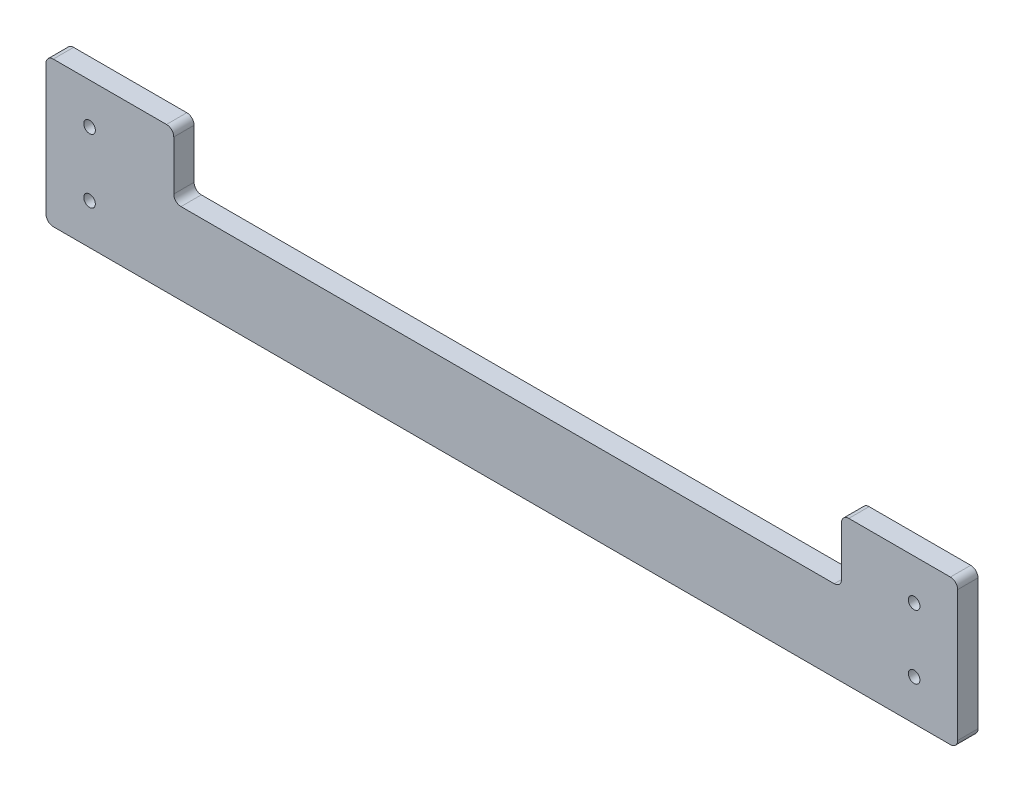
from build123d import *

# Parameters (mm, degrees)
SKETCH_1_W          = 1570
SKETCH_1_H          = 250
EXTRUDE_1_DEPTH     = 35
CUT_EXTRUDE_1_REACH = 797.66
SKETCH_2_W          = 1150
SKETCH_2_H          = 110
FILLET_1_R          = 12.5
CUT_EXTRUDE_2_REACH = 797.66
SKETCH_4_R          = 10


with BuildPart() as part:
    # 草图1 → 凸台-拉伸1 (new body)
    with BuildSketch(Plane.XY):
        Rectangle(SKETCH_1_W, SKETCH_1_H)
    extrude(amount=EXTRUDE_1_DEPTH)

    # 草图2 → 切除-拉伸1 (cut, up to next)
    with BuildSketch(Plane.XY.offset(35), mode=Mode.PRIVATE) as cut_extrude_1_sk1:
        with Locations((10, 70)):
            Rectangle(SKETCH_2_W, SKETCH_2_H)
    cut_extrude_1_tool1 = extrude(cut_extrude_1_sk1.sketch, amount=-CUT_EXTRUDE_1_REACH, mode=Mode.PRIVATE) & part.part
    add(cut_extrude_1_tool1.solids().sort_by_distance((10, 70, 35))[0], mode=Mode.SUBTRACT)

    # 圆角1
    fillet_1_edges = [part.edges().sort_by_distance(p)[0] for p in [
        (-565, 125, 17.5),
        (585, 125, 17.5),
        (585, 15, 17.5),
        (-565, 15, 17.5),
        (785, -125, 17.5),
        (-785, -125, 17.5),
        (-785, 125, 17.5),
        (785, 125, 17.5),
    ]]
    fillet(fillet_1_edges, radius=FILLET_1_R)

    # 草图4 → 切除-拉伸2 (cut, up to next)
    with BuildSketch(Plane.XY.offset(35), mode=Mode.PRIVATE) as cut_extrude_2_sk1:
        with Locations((-710, 55)):
            Circle(SKETCH_4_R)
    cut_extrude_2_tool1 = extrude(cut_extrude_2_sk1.sketch, amount=-CUT_EXTRUDE_2_REACH, mode=Mode.PRIVATE) & part.part
    # 草图4 → 切除-拉伸2 (cut, up to next)
    with BuildSketch(Plane.XY.offset(35), mode=Mode.PRIVATE) as cut_extrude_2_sk2:
        with Locations((-710, -55)):
            Circle(SKETCH_4_R)
    cut_extrude_2_tool2 = extrude(cut_extrude_2_sk2.sketch, amount=-CUT_EXTRUDE_2_REACH, mode=Mode.PRIVATE) & part.part
    # 草图4 → 切除-拉伸2 (cut, up to next)
    with BuildSketch(Plane.XY.offset(35), mode=Mode.PRIVATE) as cut_extrude_2_sk3:
        with Locations((710, 55)):
            Circle(SKETCH_4_R)
    cut_extrude_2_tool3 = extrude(cut_extrude_2_sk3.sketch, amount=-CUT_EXTRUDE_2_REACH, mode=Mode.PRIVATE) & part.part
    # 草图4 → 切除-拉伸2 (cut, up to next)
    with BuildSketch(Plane.XY.offset(35), mode=Mode.PRIVATE) as cut_extrude_2_sk4:
        with Locations((710, -55)):
            Circle(SKETCH_4_R)
    cut_extrude_2_tool4 = extrude(cut_extrude_2_sk4.sketch, amount=-CUT_EXTRUDE_2_REACH, mode=Mode.PRIVATE) & part.part
    add(cut_extrude_2_tool1.solids().sort_by_distance((-710, 55, 35))[0], mode=Mode.SUBTRACT)
    add(cut_extrude_2_tool2.solids().sort_by_distance((-710, -55, 35))[0], mode=Mode.SUBTRACT)
    add(cut_extrude_2_tool3.solids().sort_by_distance((710, 55, 35))[0], mode=Mode.SUBTRACT)
    add(cut_extrude_2_tool4.solids().sort_by_distance((710, -55, 35))[0], mode=Mode.SUBTRACT)


solid = part.part
